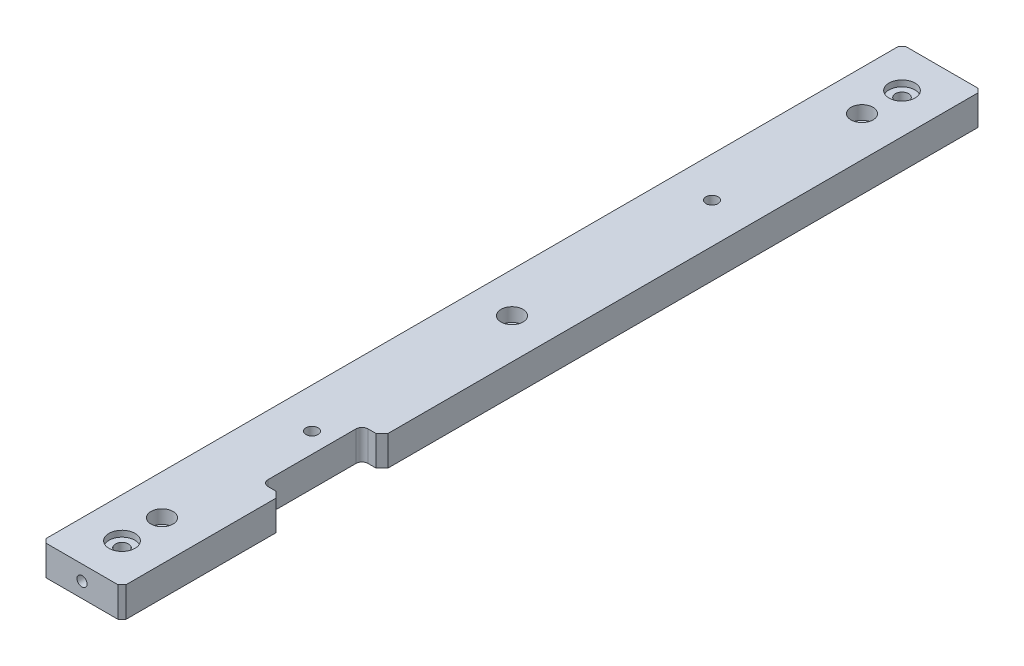
from build123d import *

# Parameters (mm, degrees)
SKETCH1_W                                    = 40
SKETCH1_H                                    = 430
BOSS_EXTRUDE1_DEPTH                          = 7.5
SKETCH2_R                                    = 6.5
CUT_EXTRUDE1_DEPTH                           = 3
HEX_SOCKET_CAP_SCREW_HOLE_TYPE_1_D           = 6.6
HEX_SOCKET_CAP_SCREW_HOLE_TYPE_1_CBORE_D     = 11
HEX_SOCKET_CAP_SCREW_HOLE_TYPE_1_CBORE_DEPTH = 6.8
M5_TAPPED_HOLE1_D                            = 4.2
M5_TAPPED_HOLE1_DEPTH                        = 15
M5_TAPPED_HOLE1_TIP                          = 1.2618073
CHAMFER1_SIZE                                = 2
HEX_SOCKET_CAP_SCREW_HOLE_TYPE_2_D           = 6.6
HEX_SOCKET_CAP_SCREW_HOLE_TYPE_2_CBORE_D     = 11
HEX_SOCKET_CAP_SCREW_HOLE_TYPE_2_CBORE_DEPTH = 6.8
M6_TAPPED_HOLE1_D                            = 5
M6_TAPPED_HOLE1_DEPTH                        = 13
M6_TAPPED_HOLE1_TIP                          = 1.502151548
M6_TAPPED_HOLE2_D                            = 5
M6_TAPPED_HOLE2_DEPTH                        = 13
M6_TAPPED_HOLE2_TIP                          = 1.502151548
F_6_0_6_DIAMETER_HOLE1_D                     = 6
F_6_0_6_DIAMETER_HOLE1_DEPTH                 = 17
F_6_0_6_DIAMETER_HOLE1_TIP                   = 1.802581857
SKETCH15_W                                   = 10
SKETCH15_H                                   = 50
CUT_EXTRUDE2_DEPTH                           = 217.448608228
FILLET1_R                                    = 3
CHAMFER2_SIZE                                = 3


with BuildPart() as part:
    # Sketch1 → Boss-Extrude1 (new, symmetric)
    with BuildSketch(Plane(origin=(0, 0, 0), x_dir=(1, 0, 0), z_dir=(0, 1, 0))):
        Rectangle(SKETCH1_W, SKETCH1_H)
    extrude(amount=BOSS_EXTRUDE1_DEPTH, both=True)

    # Sketch2 → Cut-Extrude1 (cut)
    with BuildSketch(Plane(origin=(0, 7.5, 0), x_dir=(1, 0, 0), z_dir=(0, 1, 0))):
        with Locations(Location((0, 195, 0), (0, 0, 270))):
            Circle(SKETCH2_R)
        with Locations(Location((0, -195, 0), (0, 0, 90))):
            Circle(SKETCH2_R)
    extrude(amount=-CUT_EXTRUDE1_DEPTH, mode=Mode.SUBTRACT)

    # Hex socket cap screw hole type 1 (through all)
    with Locations(Plane(origin=(0, -7.5, 0), x_dir=(-1, 0, 0), z_dir=(0, -1, 0))):
        with Locations((0, -195), (0, 195)):
            CounterBoreHole(HEX_SOCKET_CAP_SCREW_HOLE_TYPE_1_D / 2, HEX_SOCKET_CAP_SCREW_HOLE_TYPE_1_CBORE_D / 2, HEX_SOCKET_CAP_SCREW_HOLE_TYPE_1_CBORE_DEPTH)

    # M5 Tapped Hole1
    with Locations(Plane.ZY.offset(20)):
        with Locations((-195, 0), (195, 0), (-65, 0), (65, 0)):
            Hole(M5_TAPPED_HOLE1_D / 2, depth=M5_TAPPED_HOLE1_DEPTH)
            with Locations((0, 0, -(M5_TAPPED_HOLE1_DEPTH + M5_TAPPED_HOLE1_TIP / 2))):  # 118° drill point
                Cone(0, M5_TAPPED_HOLE1_D / 2, M5_TAPPED_HOLE1_TIP, mode=Mode.SUBTRACT)

    # Chamfer1
    chamfer1_edges = [part.edges().sort_by_distance(p)[0] for p in [
        (-20, 0, -215),
        (20, 0, -215),
        (20, 0, 215),
        (-20, 0, 215),
    ]]
    chamfer(chamfer1_edges, length=CHAMFER1_SIZE)

    # Hex socket cap screw hole type 2 (through all)
    with Locations(Plane(origin=(0, 7.5, 0), x_dir=(1, 0, 0), z_dir=(0, 1, 0))):
        with Locations((0, 175), (0, -175), (0, 0)):
            CounterBoreHole(HEX_SOCKET_CAP_SCREW_HOLE_TYPE_2_D / 2, HEX_SOCKET_CAP_SCREW_HOLE_TYPE_2_CBORE_D / 2, HEX_SOCKET_CAP_SCREW_HOLE_TYPE_2_CBORE_DEPTH)

    # M6 Tapped Hole1
    with Locations(Plane.XY.offset(215)):
        with Locations((0, 0)):
            Hole(M6_TAPPED_HOLE1_D / 2, depth=M6_TAPPED_HOLE1_DEPTH)
            with Locations((0, 0, -(M6_TAPPED_HOLE1_DEPTH + M6_TAPPED_HOLE1_TIP / 2))):  # 118° drill point
                Cone(0, M6_TAPPED_HOLE1_D / 2, M6_TAPPED_HOLE1_TIP, mode=Mode.SUBTRACT)

    # M6 Tapped Hole2
    with Locations(Plane(origin=(0, 0, -215), x_dir=(-1, 0, 0), z_dir=(0, 0, -1))):
        with Locations((0, 0)):
            Hole(M6_TAPPED_HOLE2_D / 2, depth=M6_TAPPED_HOLE2_DEPTH)
            with Locations((0, 0, -(M6_TAPPED_HOLE2_DEPTH + M6_TAPPED_HOLE2_TIP / 2))):  # 118° drill point
                Cone(0, M6_TAPPED_HOLE2_D / 2, M6_TAPPED_HOLE2_TIP, mode=Mode.SUBTRACT)

    # Ø6.0 (6) Diameter Hole1
    with Locations(Plane(origin=(0, -7.5, 0), x_dir=(-1, 0, 0), z_dir=(0, -1, 0))):
        with Locations((0, 100), (0, -100)):
            Hole(F_6_0_6_DIAMETER_HOLE1_D / 2, depth=F_6_0_6_DIAMETER_HOLE1_DEPTH)
            with Locations((0, 0, -(F_6_0_6_DIAMETER_HOLE1_DEPTH + F_6_0_6_DIAMETER_HOLE1_TIP / 2))):  # 118° drill point
                Cone(0, F_6_0_6_DIAMETER_HOLE1_D / 2, F_6_0_6_DIAMETER_HOLE1_TIP, mode=Mode.SUBTRACT)

    # Sketch15 → Cut-Extrude2 (cut, through all)
    with BuildSketch(Plane.XZ.offset(7.5)):
        with Locations((15, 110)):
            Rectangle(SKETCH15_W, SKETCH15_H)
    extrude(amount=-CUT_EXTRUDE2_DEPTH, mode=Mode.SUBTRACT)

    # Fillet1
    fillet1_edges = [part.edges().sort_by_distance(p)[0] for p in [
        (10, 0, 85),
        (10, 0, 135),
    ]]
    fillet(fillet1_edges, radius=FILLET1_R)

    # Chamfer2
    chamfer2_edges = [part.edges().sort_by_distance(p)[0] for p in [
        (20, 0, 135),
        (20, 0, 85),
    ]]
    chamfer(chamfer2_edges, length=CHAMFER2_SIZE)


solid = part.part
